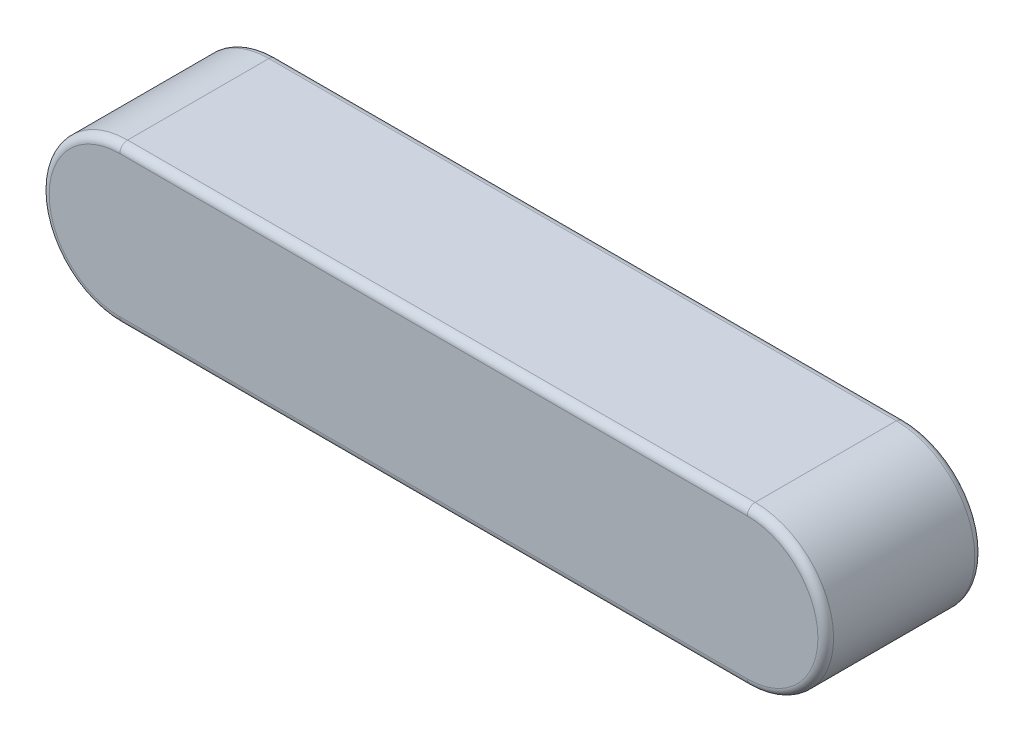
SolidWorks part; units mm, degrees
ref_plane "Plane1" through (0, 0, 0) normal (0, 0, 1) x (1, 0, 0)
ref_plane "Plane2" through (0, 0, 0) normal (0, 1, 0) x (1, 0, 0)
ref_plane "Plane3" through (0, 0, 0) normal (1, 0, 0) x (0, 0, -1)
sketch "Dimension Sketch" plane through (0, 0, 0) normal (0, 0, 1) x (1, 0, 0)
  line L0 (-12.5, 0) -> (12.5, 0) construction
  point P3 (-5, 0)
  point P4 (0, 0)
  point P5 (0.25, 0)
  point P8 (-5, 0)
  point P11 (0, 0)
  dimension "L" = 25
  dimension "b" = 5
  dimension "h" = 5
  dimension "r" = 0.25
sketch "Sketch1" plane through (0, 0, 0) normal (0, 0, 1) x (1, 0, 0)
  line L0 (-12.5, 0) -> (12.5, 0) construction
  line L1 (-10, 2.5) -> (10, 2.5)
  line L2 (-10, -2.5) -> (10, -2.5)
  line L3 (0, 2.9108) -> (0, -2.5) construction
  arc A0 (-10, 2.5) -> (-10, -2.5) centre (-10, 0) ccw
  arc A1 (10, 2.5) -> (10, -2.5) centre (10, 0) cw
  dimension "D3" = 25
  dimension "D1" = 2.5
extrude "Base-Extrude" add sketch "Sketch1" along normal blind 5
fillet "Fillet1" radius 0.25 8 edges at (12.5, 0, 5) (0, 2.5, 5) (-12.5, 0, 5) (0, 2.5, 0) (12.5, 0, 0) (0, -2.5, 0) (-12.5, 0, 0) (0, -2.5, 5)
